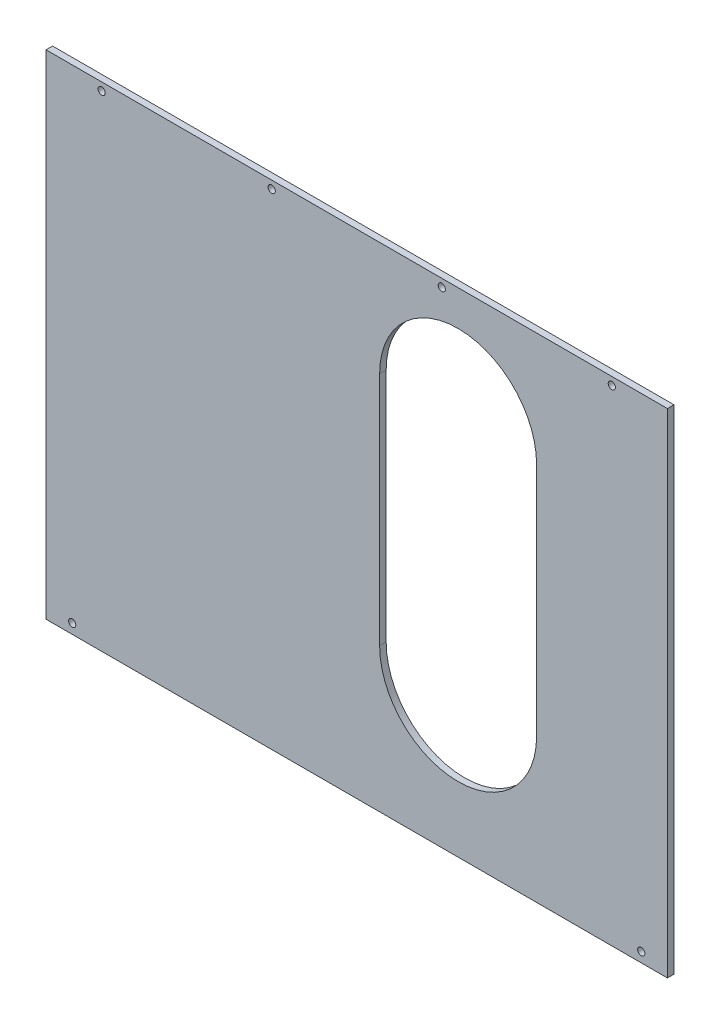
SolidWorks part; units mm, degrees
material "PC "
ref_plane "Front Plane" through (0, 0, 0) normal (0, 0, 1) x (1, 0, 0)
ref_plane "Top Plane" through (0, 0, 0) normal (0, 1, 0) x (1, 0, 0)
ref_plane "Right Plane" through (0, 0, 0) normal (1, 0, 0) x (0, 0, -1)
sketch "Sketch1" plane through (0, 0, 0) normal (0, 0, 1) x (1, 0, 0)
  line L1 (-237.5, 188.5) -> (237.5, 188.5)
  line L2 (-237.5, 188.5) -> (-237.5, -188.5)
  line L3 (-237.5, -188.5) -> (237.5, -188.5)
  line L4 (237.5, 188.5) -> (237.5, -188.5)
  line L5 (-237.5, 188.5) -> (237.5, -188.5) construction
  line L6 (-237.5, -188.5) -> (237.5, 188.5) construction
  point P0 (0, 0)
  dimension "D1" = 475
  dimension "D2" = 377
extrude "Boss-Extrude1" add sketch "Sketch1" along normal blind 5
sketch "Sketch3" plane through (0, 0, 0) normal (0, 0, -1) x (-1, 0, 0)
  line L2 (-77.5, 101.5) -> (-77.5, -78.5) construction
  line L3 (-17.5, 101.5) -> (-17.5, -78.5)
  line L4 (-137.5, 101.5) -> (-137.5, -78.5)
  line L5 (-237.5, -188.5) -> (-237.5, 188.5) construction
  line L6 (237.5, -188.5) -> (-237.5, -188.5) construction
  arc A1 (-17.5, 101.5) -> (-137.5, 101.5) centre (-77.5, 101.5) ccw
  arc A2 (-137.5, -78.5) -> (-17.5, -78.5) centre (-77.5, -78.5) ccw
  point P6 (-77.5, 11.5)
  dimension "D1" = 60
  dimension "D2" = 180
  dimension "D3" = 160
  dimension "D4" = 200
hole_wizard "M5 Clearance Hole1" positions "Sketch4" profile "Sketch5" hole size "M5" standard "GB" end condition up to next
sketch "Sketch4" plane through (0, 0, 0) normal (0, 0, -1) x (-1, 0, 0)
  point P0 (-195, 182.5)
  point P3 (-65, 182.5)
  point P6 (65, 182.5)
  point P9 (195, 182.5)
  point P12 (217.5, -181)
  point P15 (-217.5, -181)
sketch "Sketch5" plane through (195, 182.5, 0) normal (1, 0, 0) x (0, 1, 0)
  line L0 (0, 0) -> (0, 5)
  line L1 (0, 5) -> (2.75, 5)
  line L2 (2.75, 5) -> (2.75, 0)
  line L5 (2.75, 0) -> (0, 0)
  line L11 (0, -6.35) -> (0, 107.95) construction
  dimension "通孔孔直径" = 5.5
  dimension "通孔孔深度" = 5
extrude "Cut-Extrude1" cut sketch "Sketch3" against normal blind 10
